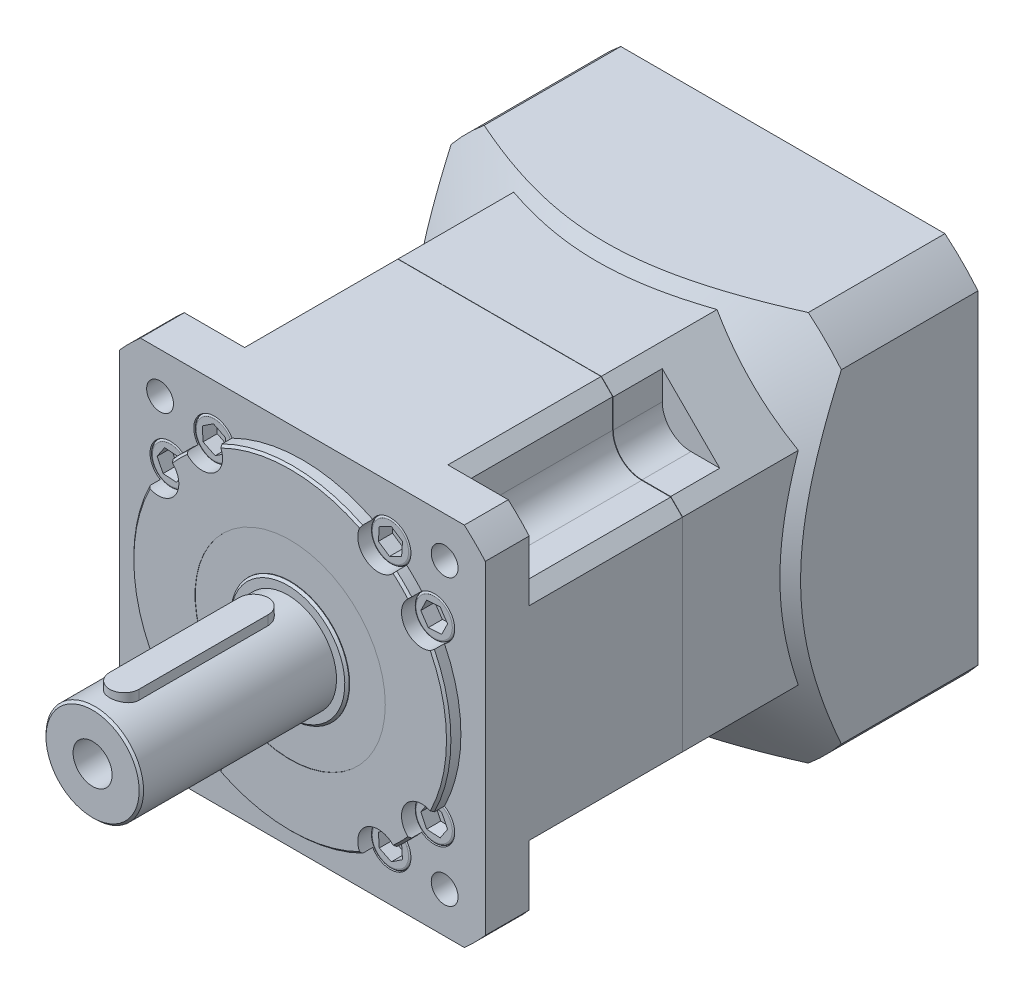
SolidWorks part; units mm, degrees
ref_plane "前视基准面" through (0, 0, 0) normal (0, 0, 1) x (1, 0, 0)
ref_plane "上视基准面" through (0, 0, 0) normal (0, 1, 0) x (1, 0, 0)
ref_plane "右视基准面" through (0, 0, 0) normal (1, 0, 0) x (0, 0, -1)
sketch "草图1" plane through (0, 0, 0) normal (1, 0, 0) x (0, 0, -1)
  line L0 (-283, 0) -> (0, 0) construction
  line L1 (-283, 0) -> (-283, 20)
  line L2 (-283, 20) -> (-203, 20)
  line L3 (-203, 20) -> (-203, 24.3)
  line L4 (-203, 24.3) -> (-202, 24.3)
  line L5 (-197, 65) -> (-197, 75)
  line L6 (-197, 75) -> (-42.45, 75)
  line L7 (0, 80) -> (0, 0)
  line L8 (-283, 8) -> (-263, 8)
  line L9 (-263, 8) -> (-258.3812, 0)
  line L10 (-202, 24.3) -> (-202, 65)
  line L11 (-202, 65) -> (-197, 65)
  line L12 (0, 55) -> (-10, 55)
  line L13 (-10, 55) -> (-10, 11)
  line L14 (-10, 11) -> (-62, 11)
  line L15 (-62, 11) -> (-62, 0)
  line L16 (-42.45, 80) -> (-42.45, 75)
  line L18 (-42.45, 80) -> (0, 80)
  point P7 (-96, 75)
  point P11 (-276, 20)
  point P13 (-211, 20)
  point P19 (-179, 75)
  point P23 (-24, 75)
  point P24 (-42.45, 75)
  point P25 (-116.2, 75)
  dimension "D1" = 60
  dimension "A1" = 283
  dimension "D2" = 16
  dimension "D3" = 20
  dimension "D4" = 40
  dimension "D5" = 7
  dimension "D6" = 65
  dimension "D7" = 80
  dimension "D8" = 5
  dimension "D9" = 86
  dimension "D10" = 48.6
  dimension "D11" = 130
  dimension "D12" = 160
  dimension "A" = 101
  dimension "D13" = 150
  dimension "C" = 110
  dimension "(d)" = 22
  dimension "D" = 10
  dimension "B" = 62
  dimension "D17" = 18
  dimension "D18" = 24
  dimension "D19" = 42.45
  dimension "D20" = 80.8
sketch "输出端" plane through (0, 0, 0) normal (0, 0, 1) x (1, 0, 0)
  line L0 (0, 75) -> (0, -75) construction
  line L1 (-75, -75) -> (75, -75)
  line L2 (-75, -75) -> (-75, 75)
  line L3 (-75, 75) -> (75, 75)
  line L4 (75, -75) -> (75, 75)
  line L5 (-75, -75) -> (75, 75) construction
  line L6 (-75, 75) -> (75, -75) construction
  line L7 (0, 0) -> (36.1121, 54.0455) construction
  line L8 (36.1121, 54.0455) -> (38.5785, 55.2618) construction
  line L9 (40.6851, 50.9899) -> (41.0449, 56.4781)
  line L10 (41.0449, 56.4781) -> (36.4718, 59.5337)
  line L11 (36.4718, 59.5337) -> (31.539, 57.1012)
  line L12 (31.539, 57.1012) -> (31.1793, 51.6129)
  line L13 (31.1793, 51.6129) -> (35.7523, 48.5573)
  line L14 (35.7523, 48.5573) -> (40.6851, 50.9899)
  line L15 (38.5785, 55.2618) -> (41.0449, 56.4781) construction
  line L16 (43.5113, 57.6944) -> (41.0449, 56.4781) construction
  line L17 (-6, 23) -> (6, 23)
  line L19 (58.3363, 58.3363) -> (66.6682, 66.6682)
  line L22 (41.6726, 75) -> (75, 41.6726)
  line L23 (66.6682, 66.6682) -> (75, 75)
  line L24 (46.5533, 58.3363) -> (46.5533, 75)
  line L25 (58.3363, 46.5533) -> (75, 46.5533)
  circle A0 centre (0, 0) radius 82.5 construction
  circle A1 centre (58.3363, 58.3363) radius 5.5
  circle A2 centre (0, 0) radius 65 construction
  circle A3 centre (36.1121, 54.0455) radius 4.7631 construction
  circle A4 centre (36.1121, 54.0455) radius 8.25
  circle A5 centre (36.1121, 54.0455) radius 8.4
  circle A6 centre (0, 0) radius 20
  circle A7 centre (58.3363, 58.3363) radius 11.783
  circle A8 centre (0, 0) radius 39
  circle A9 centre (0, 0) radius 24.3
  circle A10 centre (0, 0) radius 100.1745
  point P0 (0, 0)
  point P30 (0, 23)
  point P31 (0, -20)
  point P35 (70.8341, 70.8341)
  dimension "D1" = 165
  dimension "D2" = 11
  dimension "D3" = 0.15
  dimension "D4" = 16.5
  dimension "D8" = 78
  dimension "D5" = 33.75
  dimension "D6" = 43
  dimension "D7" = 12
sketch "输入端" plane through (0, 0, 0) normal (0, 0, 1) x (1, 0, 0)
  line L0 (0, 80) -> (0, -80) construction
  line L1 (-80, -80) -> (80, -80)
  line L2 (-80, -80) -> (-80, 80)
  line L3 (-80, 80) -> (80, 80)
  line L4 (80, -80) -> (80, 80)
  line L5 (-80, -80) -> (80, 80) construction
  line L6 (-80, 80) -> (80, -80) construction
  line L7 (0, 0) -> (-21.0476, 50.8134) construction
  line L8 (-21.0476, 50.8134) -> (-20.7865, 52.7963) construction
  line L9 (-20.5255, 54.7792) -> (-24.221, 53.2484)
  line L10 (-24.221, 53.2484) -> (-24.7431, 49.2826)
  line L11 (-24.7431, 49.2826) -> (-21.5697, 46.8476)
  line L12 (-21.5697, 46.8476) -> (-17.8742, 48.3783)
  line L13 (-17.8742, 48.3783) -> (-17.3521, 52.3441)
  line L14 (-17.3521, 52.3441) -> (-20.5255, 54.7792)
  line L15 (-20.7865, 52.7963) -> (-20.5255, 54.7792) construction
  line L16 (-20.2644, 56.762) -> (-20.5255, 54.7792) construction
  circle A0 centre (0, 0) radius 72.5 construction
  circle A1 centre (51.2652, 51.2652) radius 4
  circle A2 centre (0, 0) radius 11
  circle A3 centre (0, 0) radius 55
  circle A4 centre (-21.0476, 50.8134) radius 3.4641 construction
  circle A5 centre (-21.0476, 50.8134) radius 6
  circle A6 centre (-21.0476, 50.8134) radius 6.15
  circle A7 centre (0, 0) radius 33
  circle A8 centre (0, 0) radius 104
  point P0 (0, 0)
  dimension "D1" = 0.15
  dimension "F" = 145
  dimension "D2" = 22.5
  dimension "E" = 8
  dimension "D3" = 12
  dimension "D4" = 66
  dimension "D5" = 208
sketch "草图4" plane through (0, 0, 0) normal (1, 0, 0) x (0, 0, -1)
  line L0 (-202, 65) -> (-197, 65) construction
  line L1 (-202, 24.3) -> (-202, 65) construction
  line L2 (-203, 20) -> (-203, 24.3) construction
  line L3 (-203, 24.3) -> (-202, 24.3) construction
  line L4 (-283, 20) -> (-203, 20) construction
  line L5 (-283, 0) -> (-283, 20) construction
  line L6 (-283, 8) -> (-263, 8) construction
  line L7 (-263, 8) -> (-258.3812, 0) construction
  line L8 (-202, 65) -> (-197, 65)
  line L9 (-202, 24.3) -> (-202, 65)
  line L10 (-203, 20) -> (-203, 24.3)
  line L11 (-203, 24.3) -> (-202, 24.3)
  line L12 (-283, 20) -> (-203, 20)
  line L13 (-283, 8) -> (-283, 20)
  line L14 (-283, 8) -> (-263, 8)
  line L15 (-263, 8) -> (-258.3812, 0)
  line L16 (-197, 65) -> (-197, 0)
  line L17 (-197, 0) -> (-258.3812, 0)
revolve "旋转1" add sketch "草图4" angle 360 mid plane about L17
cosmetic thread "装饰螺纹线2" parameters "D2"=16.1
sketch "草图15" plane through (0, 0, 0) normal (0, 1, 0) x (1, 0, 0)
  line L0 (0, -270) -> (0, -217) construction
  line L1 (0, -283) -> (0, -263) construction
  line L2 (-6, -270) -> (-6, -217)
  line L3 (6, -270) -> (6, -217)
  line L4 (0, -283) -> (0, 0) construction
  arc A0 (-6, -270) -> (6, -270) centre (0, -270) ccw
  arc A1 (6, -217) -> (-6, -217) centre (0, -217) ccw
  point P4 (0, -243.5)
  point P9 (0, -276)
  point P10 (0, -211)
extrude "凸台-拉伸2" add sketch "草图15" along normal up to vertex (23 mm away) from vertex at 8 starting at point (0, 8, 283)
chamfer "倒角1" distance 0.9 angle 45 3 edges at (0, 65, 202) (0, 24.3, 203) (0, 20, 283)
sketch "草图6" plane through (0, 0, 0) normal (0, 0, 1) x (1, 0, 0)
  line L0 (-75, 75) -> (75, 75) construction
  line L1 (-75, -75) -> (-75, 75) construction
  line L2 (-75, -75) -> (75, -75) construction
  line L3 (75, -75) -> (75, 75) construction
  line L4 (-75, 75) -> (75, 75)
  line L5 (-75, -75) -> (-75, 75)
  line L6 (-75, -75) -> (75, -75)
  line L7 (75, -75) -> (75, 75)
extrude "凸台-拉伸1" add sketch "草图6" along normal up to vertex (197 mm away) from vertex at 42.45 starting at point (0, 75, 42.45)
sketch "草图7" plane through (0, 0, 197) normal (0, 0, 1) x (1, 0, 0)
  line L2 (66.4073, 75) -> (75, 75)
  line L3 (75, -75) -> (75, 75) construction
  line L4 (75, 75) -> (-75, 75) construction
  line L5 (75, 75) -> (75, 66.4073)
  circle A0 centre (58.3363, 58.3363) radius 5.5 construction
  circle A1 centre (58.3363, 58.3363) radius 5.5
  circle A2 centre (0, 0) radius 100.1745 construction
  arc A3 (75, 66.4073) -> (66.4073, 75) centre (0, 0) ccw
extrude "切除-拉伸1" cut sketch "草图7" against normal up to vertex (18 mm away) up to point (0, 75, 179)
sketch "草图9" plane through (0, 0, 0) normal (0, 0, 1) x (1, 0, 0)
  line L0 (41.6726, 75) -> (75, 41.6726) construction
  line L1 (41.6726, 75) -> (75, 41.6726)
  line L2 (41.6726, 75) -> (75, 75)
  line L3 (75, 75) -> (75, 41.6726)
extrude "切除-拉伸3" cut sketch "草图9" against normal up to vertex (-42.45 mm away) from vertex at 179 starting at point (0, 75, 179)
sketch "草图8" plane through (0, 0, 0) normal (0, 0, 1) x (1, 0, 0)
  line L2 (58.3363, 46.5533) -> (75, 46.5533) construction
  line L3 (46.5533, 58.3363) -> (46.5533, 75) construction
  line L4 (58.3363, 46.5533) -> (75, 46.5533)
  line L5 (46.5533, 58.3363) -> (46.5533, 75)
  line L6 (46.5533, 75) -> (75, 75)
  line L7 (75, 75) -> (75, 46.5533)
  circle A1 centre (58.3363, 58.3363) radius 11.783 construction
  arc A2 (46.5533, 58.3363) -> (58.3363, 46.5533) centre (58.3363, 58.3363) ccw
extrude "切除-拉伸2" cut sketch "草图8" against normal up to vertex (-96 mm away) from vertex at 179 starting at point (0, 75, 179)
sketch "草图10" plane through (0, 0, 179) normal (0, 0, -1) x (-1, 0, 0)
  line L0 (-46.5533, 70.1193) -> (-46.5533, 58.3363) construction
  line L1 (-58.3363, 46.5533) -> (-70.1193, 46.5533) construction
  line L2 (-46.5533, 70.1193) -> (-46.5533, 58.3363)
  line L3 (-58.3363, 46.5533) -> (-70.1193, 46.5533)
  line L4 (-46.4533, 70.2193) -> (-46.4533, 58.3363)
  line L5 (-58.3363, 46.4533) -> (-70.2193, 46.4533)
  line L6 (-46.5533, 70.1193) -> (-46.4533, 70.2193)
  line L7 (-41.6726, 75) -> (-46.5533, 70.1193) construction
  line L8 (-46.4533, 70.1193) -> (-46.4533, 58.3363) construction
  line L9 (-58.3363, 46.4533) -> (-70.1193, 46.4533) construction
  line L10 (-70.1193, 46.5533) -> (-70.2193, 46.4533)
  line L11 (-70.1193, 46.5533) -> (-75, 41.6726) construction
  arc A0 (-58.3363, 46.5533) -> (-46.5533, 58.3363) centre (-58.3363, 58.3363) ccw construction
  arc A1 (-58.3363, 46.5533) -> (-46.5533, 58.3363) centre (-58.3363, 58.3363) ccw
  arc A2 (-58.3363, 46.4533) -> (-46.4533, 58.3363) centre (-58.3363, 58.3363) ccw
  dimension "D1" = 0.1
extrude "切除-拉伸4" cut sketch "草图10" along normal up to vertex (62.8 mm away) up to point (0, 75, 116.2)
pattern_circular "阵列(圆周)1" count 4 over 360 about axis through (0, 0, 0) along (0, 0, 1) of "切除-拉伸4", "切除-拉伸2", "切除-拉伸3", "切除-拉伸1"
sketch "草图11" plane through (0, 0, 202) normal (0, 0, 1) x (1, 0, 0)
  circle A0 centre (36.1121, 54.0455) radius 8.4 construction
  circle A1 centre (36.1121, 54.0455) radius 8.4
extrude "切除-拉伸5" cut sketch "草图11" against normal up to vertex (5 mm away) up to point (0, 65, 197)
sketch "草图12" plane through (0, 0, 0) normal (0, 0, 1) x (1, 0, 0)
  circle A0 centre (36.1121, 54.0455) radius 8.25 construction
  circle A1 centre (36.1121, 54.0455) radius 8.4 construction
  circle A2 centre (36.1121, 54.0455) radius 8.25
  circle A3 centre (36.1121, 54.0455) radius 8.4
extrude "切除-拉伸6" cut sketch "草图12" against normal blind 9.9 from vertex at 197 starting at point (0, 75, 197)
sketch "草图13" plane through (0, 0, 0) normal (0, 0, 1) x (1, 0, 0)
  line L0 (40.6851, 50.9899) -> (41.0449, 56.4781) construction
  line L1 (41.0449, 56.4781) -> (36.4718, 59.5337) construction
  line L2 (36.4718, 59.5337) -> (31.539, 57.1012) construction
  line L3 (31.539, 57.1012) -> (31.1793, 51.6129) construction
  line L4 (31.1793, 51.6129) -> (35.7523, 48.5573) construction
  line L5 (35.7523, 48.5573) -> (40.6851, 50.9899) construction
  line L6 (40.6851, 50.9899) -> (41.0449, 56.4781)
  line L7 (41.0449, 56.4781) -> (36.4718, 59.5337)
  line L8 (36.4718, 59.5337) -> (31.539, 57.1012)
  line L9 (31.539, 57.1012) -> (31.1793, 51.6129)
  line L10 (31.1793, 51.6129) -> (35.7523, 48.5573)
  line L11 (35.7523, 48.5573) -> (40.6851, 50.9899)
extrude "切除-拉伸7" cut sketch "草图13" against normal blind 5.775 from vertex at 197 starting at point (0, 75, 197)
fillet "圆角1" radius 0.825 1 edges at (44.3621, 54.0455, 197)
pattern_circular "阵列(圆周)2" count 16 over 360 about axis through (0, 0, 0) along (0, 0, 1) skipping 2, 3, 6, 7, 10, 11, 14, 15 of "圆角1", "切除-拉伸7", "切除-拉伸5", "切除-拉伸6"
sketch "草图14" plane through (0, 0, 0) normal (0, 0, 1) x (1, 0, 0)
  circle A0 centre (0, 0) radius 39 construction
  circle A1 centre (0, 0) radius 24.3 construction
  circle A2 centre (0, 0) radius 39
  circle A3 centre (0, 0) radius 24.3
extrude "切除-拉伸8" cut sketch "草图14" against normal blind 0.1 from vertex at 202 starting at point (0, 24.3, 202)
sketch "草图16" plane through (0, 0, 0) normal (0, 0, 1) x (1, 0, 0)
  line L0 (80, -80) -> (80, 80) construction
  line L1 (-80, -80) -> (80, -80) construction
  line L2 (-80, -80) -> (-80, 80) construction
  line L3 (-80, 80) -> (80, 80) construction
  line L4 (80, -66.453) -> (80, 66.453)
  line L5 (-66.453, -80) -> (66.453, -80)
  line L6 (-80, -66.453) -> (-80, 66.453)
  line L7 (-66.453, 80) -> (66.453, 80)
  circle A0 centre (0, 0) radius 104 construction
  arc A1 (-66.453, 80) -> (-80, 66.453) centre (0, 0) ccw
  arc A2 (80, 66.453) -> (66.453, 80) centre (0, 0) ccw
  arc A3 (66.453, -80) -> (80, -66.453) centre (0, 0) ccw
  arc A4 (-80, -66.453) -> (-66.453, -80) centre (0, 0) ccw
extrude "凸台-拉伸3" add sketch "草图16" along normal up to vertex (42.45 mm away) up to point (0, 75, 42.45)
sketch "草图17" plane through (0, 0, 0) normal (0, 0, 1) x (1, 0, 0)
  circle A0 centre (51.2652, 51.2652) radius 4 construction
  circle A1 centre (51.2652, 51.2652) radius 4
extrude "切除-拉伸9" cut sketch "草图17" along normal up to vertex (24 mm away) up to point (0, 75, 24)
cosmetic thread "装饰螺纹线1" parameters "D2"=8.1
pattern_circular "阵列(圆周)3" count 4 over 360 about axis through (0, 0, 0) along (0, 0, 1) of "切除-拉伸9"
sketch "草图26" plane through (0, 0, 0) normal (1, 0, 0) x (0, 0, -1)
  line L0 (-24, 150) -> (-24, 0)
  line L2 (-24, 150) -> (-128.4016, 0)
  line L3 (-283, 0) -> (0, 0) construction
  line L4 (-128.4016, 0) -> (-24, 0)
  point P3 (-24, 75)
revolve "旋转2" add sketch "草图26" angle 360 about L4
sketch "草图27" plane through (0, 0, 0) normal (0, 0, -1) x (-1, 0, 0)
  line L0 (-66.453, 80) -> (66.453, 80) construction
  line L1 (-80, -66.453) -> (-80, 66.453) construction
  line L2 (66.453, -80) -> (-66.453, -80) construction
  line L3 (80, 66.453) -> (80, -66.453) construction
  line L4 (-66.453, 80) -> (66.453, 80)
  line L5 (-80, -66.453) -> (-80, 66.453)
  line L6 (66.453, -80) -> (-66.453, -80)
  line L7 (80, 66.453) -> (80, -66.453)
  arc A0 (-66.453, 80) -> (-80, 66.453) centre (0, 0) ccw construction
  circle A1 centre (0, 0) radius 150
  circle A2 centre (0, 0) radius 150
  arc A3 (-80, -66.453) -> (-66.453, -80) centre (0, 0) ccw construction
  arc A4 (80, 66.453) -> (66.453, 80) centre (0, 0) ccw construction
  arc A5 (66.453, -80) -> (80, -66.453) centre (0, 0) ccw construction
  arc A6 (-66.453, 80) -> (-80, 66.453) centre (0, 0) ccw
  arc A7 (-80, -66.453) -> (-66.453, -80) centre (0, 0) ccw
  arc A8 (80, 66.453) -> (66.453, 80) centre (0, 0) ccw
  arc A9 (66.453, -80) -> (80, -66.453) centre (0, 0) ccw
  dimension "D1" = 0
extrude "切除-拉伸15" cut sketch "草图27" against normal up to vertex (96 mm away) up to point (0, 75, 96)
sketch "草图20" plane through (0, 0, 0) normal (1, 0, 0) x (0, 0, -1)
  line L0 (0, 55) -> (-10, 55) construction
  line L1 (-10, 55) -> (-10, 11) construction
  line L2 (-10, 11) -> (-62, 11) construction
  line L3 (-62, 11) -> (-62, 0) construction
  line L4 (0, 55) -> (-10, 55)
  line L5 (-10, 55) -> (-10, 11)
  line L6 (-10, 11) -> (-62, 11)
  line L7 (-62, 11) -> (-62, 0)
  line L8 (0, 55) -> (0, 0)
  line L9 (0, 0) -> (-62, 0)
revolve "切除-旋转1" cut sketch "草图20" angle 360 mid plane about L9
sketch "草图21" plane through (0, 0, 0) normal (0, 0, 1) x (1, 0, 0)
  circle A0 centre (-21.0476, 50.8134) radius 6.15 construction
  circle A1 centre (-21.0476, 50.8134) radius 6.15
extrude "切除-拉伸10" cut sketch "草图21" along normal up to vertex (10 mm away) up to point (0, 55, 10)
sketch "草图22" plane through (0, 0, 0) normal (0, 0, 1) x (1, 0, 0)
  circle A0 centre (-21.0476, 50.8134) radius 6 construction
  circle A1 centre (-21.0476, 50.8134) radius 6.15 construction
  circle A2 centre (-21.0476, 50.8134) radius 6
  circle A3 centre (-21.0476, 50.8134) radius 6.15
extrude "切除-拉伸12" cut sketch "草图22" along normal blind 7.2 from vertex at 10 starting at point (0, 55, 10)
sketch "草图23" plane through (0, 0, 0) normal (0, 0, 1) x (1, 0, 0)
  line L0 (-20.5255, 54.7792) -> (-24.221, 53.2484) construction
  line L1 (-24.221, 53.2484) -> (-24.7431, 49.2826) construction
  line L2 (-24.7431, 49.2826) -> (-21.5697, 46.8476) construction
  line L3 (-21.5697, 46.8476) -> (-17.8742, 48.3783) construction
  line L4 (-17.8742, 48.3783) -> (-17.3521, 52.3441) construction
  line L5 (-17.3521, 52.3441) -> (-20.5255, 54.7792) construction
  line L6 (-20.5255, 54.7792) -> (-24.221, 53.2484)
  line L7 (-24.221, 53.2484) -> (-24.7431, 49.2826)
  line L8 (-24.7431, 49.2826) -> (-21.5697, 46.8476)
  line L9 (-21.5697, 46.8476) -> (-17.8742, 48.3783)
  line L10 (-17.8742, 48.3783) -> (-17.3521, 52.3441)
  line L11 (-17.3521, 52.3441) -> (-20.5255, 54.7792)
extrude "切除-拉伸13" cut sketch "草图23" along normal blind 4.2 from vertex at 10 starting at point (0, 55, 10)
fillet "圆角2" radius 0.6 1 edges at (-15.0476, 50.8134, 10)
pattern_circular "阵列(圆周)4" count 4 over 360 about axis through (0, 0, 0) along (0, 0, 1) of "圆角2", "切除-拉伸13", "切除-拉伸12", "切除-拉伸10"
sketch "草图24" plane through (0, 0, 0) normal (0, 0, 1) x (1, 0, 0)
  line L0 (0, 55) -> (0, -55) construction
  line L1 (0.25, 32.9991) -> (0.25, 10.9972)
  line L2 (-0.25, 32.9991) -> (-0.25, 10.9972)
  line L3 (0.25, -10.9972) -> (0.25, -32.9991)
  line L4 (-0.25, -10.9972) -> (-0.25, -32.9991)
  circle A0 centre (0, 0) radius 33 construction
  circle A1 centre (0, 0) radius 11 construction
  arc A2 (-0.25, 32.9991) -> (-0.25, -32.9991) centre (0, 0) ccw
  arc A3 (-0.25, 10.9972) -> (-0.25, -10.9972) centre (0, 0) ccw
  arc A4 (0.25, -32.9991) -> (0.25, 32.9991) centre (0, 0) ccw
  arc A5 (0.25, -10.9972) -> (0.25, 10.9972) centre (0, 0) ccw
  circle A6 centre (0, 0) radius 55 construction
  circle A7 centre (0, 0) radius 55 construction
  dimension "D1" = 0.5
extrude "凸台-拉伸4" add sketch "草图24" against normal blind 1 from vertex at 10 starting at point (0, 55, 10)
sketch "草图25" plane through (0, 75, 0) normal (0, 1, 0) x (1, 0, 0)
  line L0 (-75, -116.2) -> (75, -116.2)
  line L1 (-75, 0) -> (75, 0) construction
  line L2 (-75, -116.2) -> (-75, -116.1)
  line L3 (-75, -116.1) -> (75, -116.1)
  line L4 (75, -116.1) -> (75, -116.2)
  dimension "D1" = 0.1
extrude "切除-拉伸14" cut sketch "草图25" against normal up to vertex (150 mm away) up to point (75, -75, 0)
